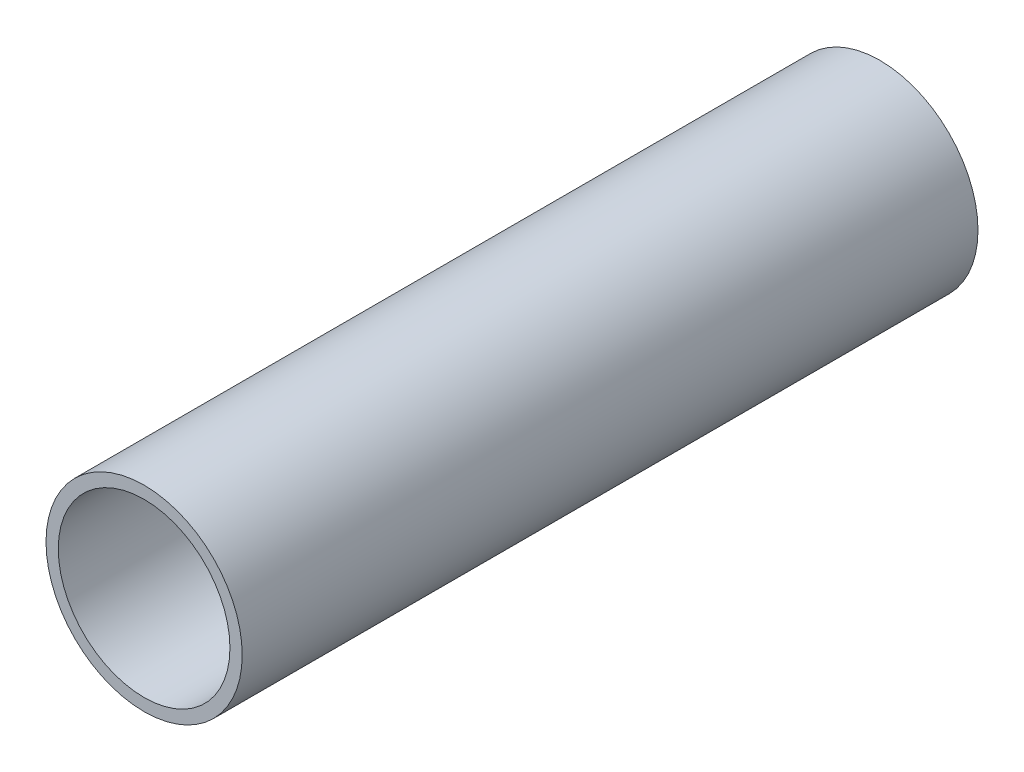
SolidWorks part; units mm, degrees
ref_plane "Front Plane" through (0, 0, 0) normal (0, 0, 1) x (1, 0, 0)
ref_plane "Top Plane" through (0, 0, 0) normal (0, 1, 0) x (1, 0, 0)
ref_plane "Right Plane" through (0, 0, 0) normal (1, 0, 0) x (0, 0, -1)
sketch "Sketch1" plane through (0, 0, 0) normal (0, 0, 1) x (1, 0, 0)
  circle A0 centre (0, 0) radius 12.6
  circle A1 centre (0, 0) radius 14.4
  dimension "D1" = 28.8
  dimension "D2" = 25.2
extrude "Boss-Extrude1" add sketch "Sketch1" along normal blind 108
